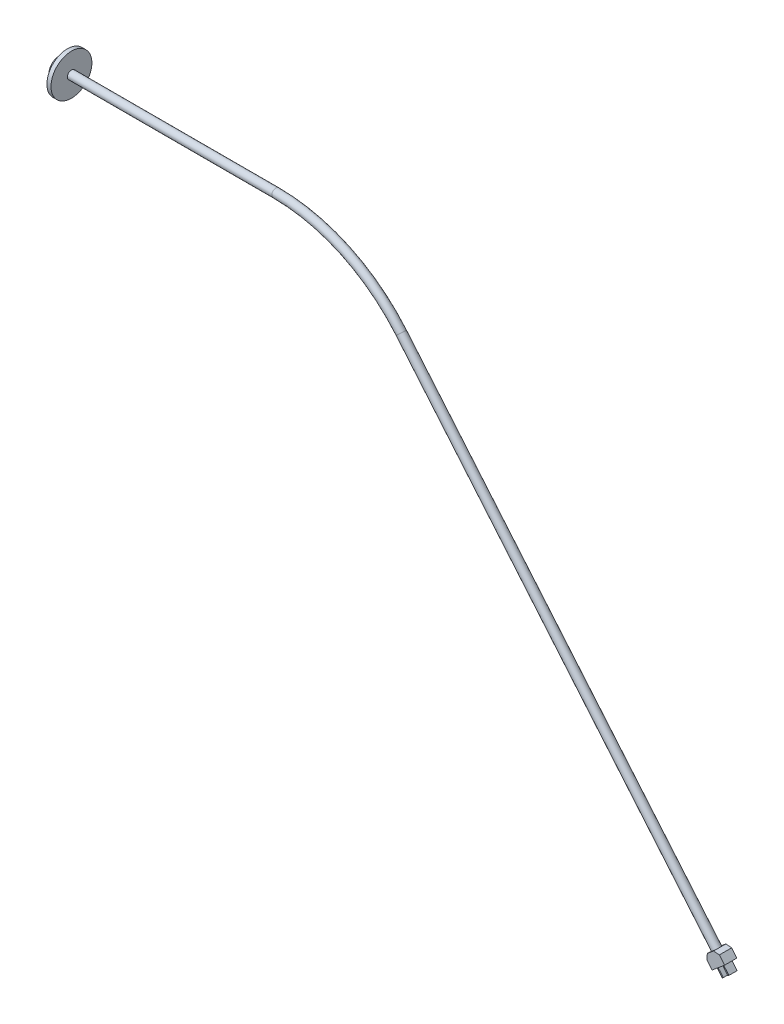
SolidWorks part; units mm, degrees
ref_plane "Front Plane" through (0, 0, 0) normal (0, 0, 1) x (1, 0, 0)
ref_plane "Top Plane" through (0, 0, 0) normal (0, 1, 0) x (1, 0, 0)
ref_plane "Right Plane" through (0, 0, 0) normal (1, 0, 0) x (0, 0, -1)
sketch "Sketch1" plane through (0, 0, 0) normal (0, 0, 1) x (1, 0, 0)
  line L0 (0, 0) -> (0, 2.5)
  line L1 (0, 2.5) -> (2, 2.5)
  line L2 (2, 2.5) -> (2, 5)
  line L3 (2, 5) -> (3, 5)
  line L4 (3, 5) -> (3, 0)
  line L5 (0, 0) -> (8.8488, 0) construction
  line L6 (0, 0) -> (3, 0)
  dimension "D1" = 5
  dimension "D2" = 2
  dimension "D3" = 10
  dimension "D4" = 1
revolve "Revolve1" add sketch "Sketch1" angle 360 about L5
sketch "Sketch2" plane through (0, 0, 0) normal (0, 0, 1) x (1, 0, 0)
  line L0 (3, 0) -> (53, 0)
  line L1 (3, -5) -> (3, 5) construction
  line L2 (83.6418, -14.2885) -> (160.7763, -106.2138)
  arc A0 (53, 0) -> (83.6418, -14.2885) centre (53, -40) cw
  dimension "D2" = 40
  dimension "D1" = 50
  dimension "D3" = 120
  dimension "D4" = 130
sweep "Sweep1" add path "Sketch2" circular profile diameter 2 parameters "D3"=2
sketch "Sketch11" plane through (0, 0, 0) normal (0, 0, 1) x (1, 0, 0)
  line L0 (160.0102, -106.8566) -> (161.5423, -105.571)
  line L1 (160.0102, -106.8566) -> (161.5423, -105.571) construction
  line L2 (161.5423, -105.571) -> (162.9512, -105.6943)
  line L3 (162.9512, -105.6943) -> (164.2367, -107.2264)
  line L4 (164.2367, -107.2264) -> (161.1726, -109.7975)
  line L5 (162.7047, -108.512) -> (160.7763, -106.2138) construction
  line L6 (159.887, -108.2654) -> (161.1726, -109.7975)
  line L7 (160.0102, -106.8566) -> (159.887, -108.2654)
  dimension "D1" = 4
  dimension "D2" = 2
  dimension "D3" = 3
extrude "Boss-Extrude1" add sketch "Sketch11" along normal mid plane 3
sketch "Sketch12" plane through (0, 0, 0) normal (0, 0, 1) x (1, 0, 0)
  line L0 (163.509, -107.837) -> (164.7946, -109.3691)
  line L1 (161.1726, -109.7975) -> (164.2367, -107.2264) construction
  line L2 (164.7946, -109.3691) -> (164.5648, -109.562)
  line L3 (164.5648, -109.562) -> (163.2792, -108.0299)
  line L4 (163.2792, -108.0299) -> (163.509, -107.837)
  line L5 (162.7047, -108.512) -> (160.7763, -106.2138) construction
  line L6 (161.5423, -105.571) -> (160.0102, -106.8566) construction
  line L7 (162.1301, -108.9941) -> (161.9003, -109.1869)
  line L8 (163.4157, -110.5261) -> (162.1301, -108.9941)
  line L9 (163.1859, -110.719) -> (163.4157, -110.5261)
  line L10 (161.9003, -109.1869) -> (163.1859, -110.719)
  dimension "D1" = 1.5
  dimension "D2" = 0.3
  dimension "D3" = 2
extrude "Boss-Extrude2" add sketch "Sketch12" along normal mid plane 2
